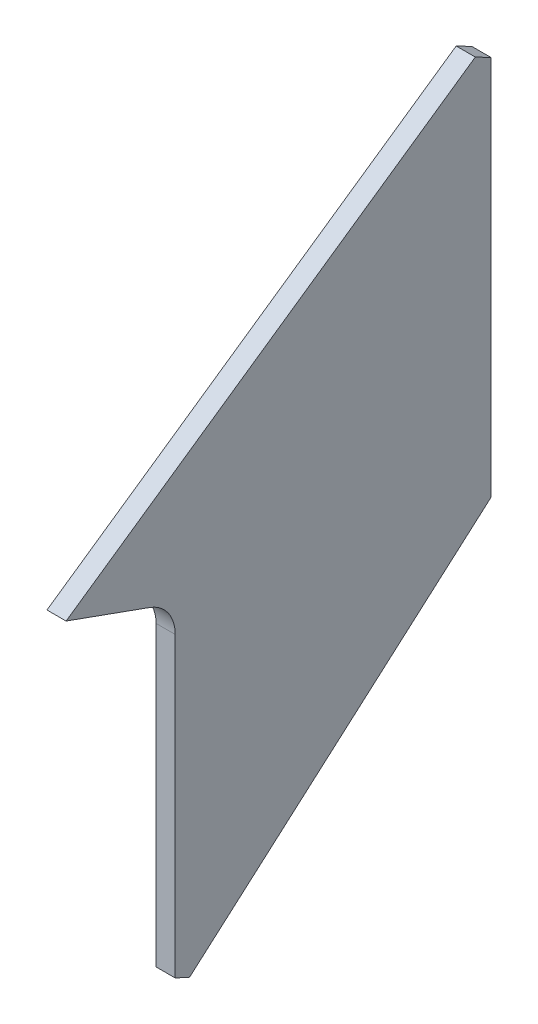
from build123d import *

# Parameters (mm, degrees)
BOSS_EXTRUDE1_DEPTH = 10


with BuildPart() as part:
    # Sketch1 → Boss-Extrude1 (new body)
    with BuildSketch(Plane(origin=(0, 0, 0), x_dir=(0, 0, -1), z_dir=(1, 0, 0))):
        with BuildLine():
            Line((0, 145), (0, 344))
            Line((0, 344), (-8.216588633, 348.300204281))
            Line((-8.216588633, 348.300204281), (-222, 200))
            Line((-222, 200), (-178.231456798, 184.258681831))
            ThreePointArc((-178.231456798, 184.258681831), (-168.638904926, 176.941636961), (-165, 165.43883))
            Line((-165, 165.43883), (-165, 10))
            Line((-165, 10), (-157.488351016, 6.601146077))
            Line((-157.488351016, 6.601146077), (0, 145))
        make_face()
    extrude(amount=BOSS_EXTRUDE1_DEPTH)


solid = part.part
